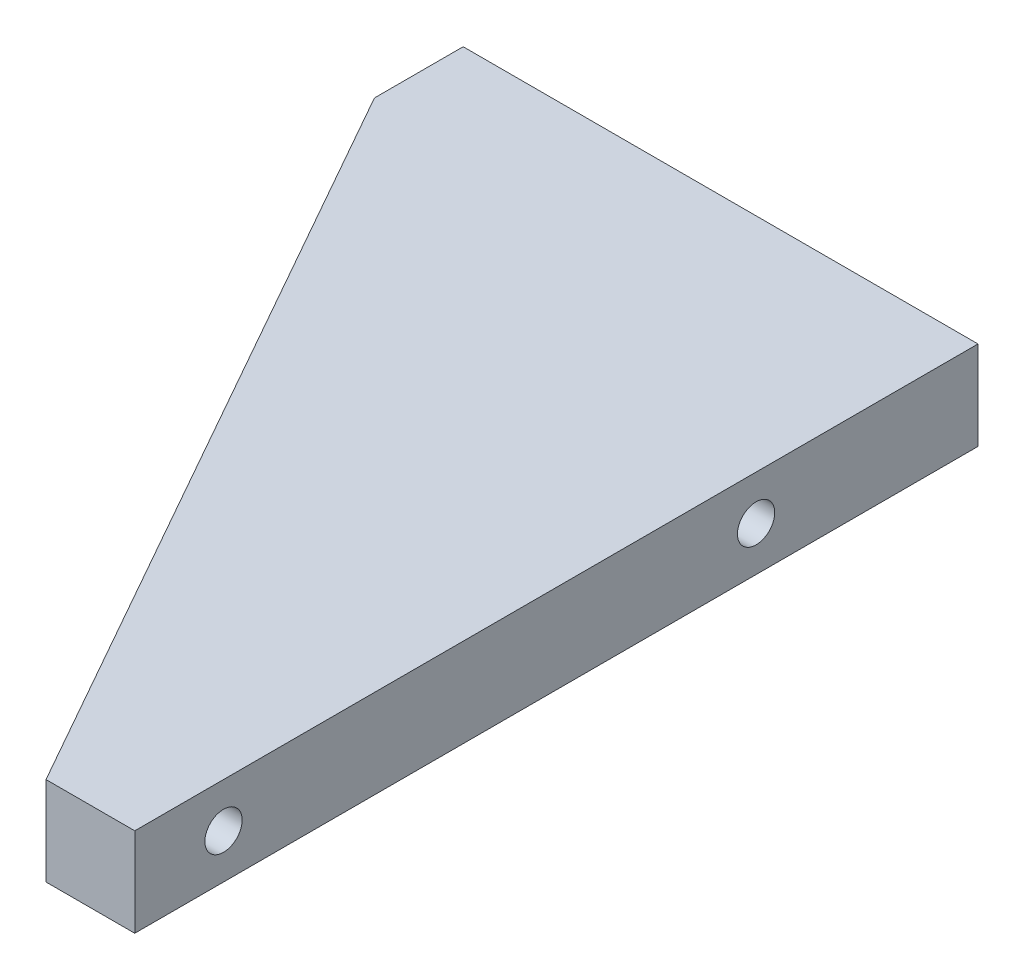
SolidWorks part; units mm, degrees
material "A6061"
ref_plane "前基準面" through (0, 0, 0) normal (0, 0, 1) x (1, 0, 0)
ref_plane "上基準面" through (0, 0, 0) normal (0, 1, 0) x (1, 0, 0)
ref_plane "右基準面" through (0, 0, 0) normal (1, 0, 0) x (0, 0, -1)
sketch "草图1" plane through (0, 0, 0) normal (0, 1, 0) x (1, 0, 0)
  line L1 (-29, -47.5) -> (29, -47.5)
  line L2 (-29, -47.5) -> (-29, 47.5)
  line L3 (-29, 47.5) -> (29, 47.5)
  line L4 (29, -47.5) -> (29, 47.5)
  line L5 (-29, -47.5) -> (29, 47.5) construction
  line L6 (-29, 47.5) -> (29, -47.5) construction
  point P0 (0, 0)
  dimension "D1" = 58
  dimension "D2" = 95
extrude "凸台-拉伸1" add sketch "草图1" along normal mid plane 10
sketch "草图2" plane through (0, 5, 0) normal (0, 1, 0) x (1, 0, 0)
  line L0 (19, -47.5) -> (-29, 37.5)
  line L1 (-29, -47.5) -> (29, -47.5) construction
  line L2 (-29, 47.5) -> (-29, -47.5) construction
  line L3 (-29, 37.5) -> (-29, -47.5)
  line L4 (-29, -47.5) -> (19, -47.5)
  line L5 (29, -47.5) -> (29, 47.5) construction
  line L6 (29, 47.5) -> (-29, 47.5) construction
  dimension "D1" = 10
  dimension "D2" = 10
extrude "切除-拉伸1" cut sketch "草图2" against normal up to surface (10 mm away) up to face at (0, -5, 0)
hole_wizard "M5 螺纹孔1" positions "草图3" profile "草图4" tap size "M5" standard "GB"
sketch "草图3" plane through (29, 0, 0) normal (1, 0, 0) x (0, 0, -1)
  line L0 (-47.5, 5) -> (-47.5, -5) construction
  point P0 (-37.5, 0)
  point P5 (22.5, 0)
  dimension "D2" = 10
  dimension "D3" = 60
  dimension "D1" = 2
sketch "草图4" plane through (29, 0, 37.5) normal (0, 1, 0) x (0, 0, -1)
  line L0 (0, 0) -> (0, 13.6618)
  line L1 (0, 13.6618) -> (2.1, 12.4)
  line L2 (2.1, 12.4) -> (2.1, 0)
  line L5 (2.1, 0) -> (0, 0)
  line L10 (0, 13.6618) -> (-2.1, 12.4) construction
  line L11 (0, -6.35) -> (0, 107.95) construction
  dimension "螺纹孔钻头直径" = 4.2
  dimension "螺纹孔钻头深度" = 12.4
  dimension "导头角度" = 118
cosmetic thread "孔螺蚊线1" parameters "D1"=10, "D2"=5
cosmetic thread "孔螺蚊线2" parameters "D1"=10, "D2"=5
hole_wizard "M5 螺纹孔2" positions "草图5" profile "草图6" tap size "M5" standard "GB"
sketch "草图5" plane through (0, 0, -47.5) normal (0, 0, -1) x (-1, 0, 0)
  line L0 (29, 5) -> (29, -5) construction
  point P0 (19, 0)
  point P2 (-21, 0)
  dimension "D1" = 40
  dimension "D2" = 10
sketch "草图6" plane through (-19, 0, -47.5) normal (1, 0, 0) x (0, 1, 0)
  line L0 (0, 0) -> (0, 13.6618)
  line L1 (0, 13.6618) -> (2.1, 12.4)
  line L2 (2.1, 12.4) -> (2.1, 0)
  line L5 (2.1, 0) -> (0, 0)
  line L10 (0, 13.6618) -> (-2.1, 12.4) construction
  line L11 (0, -6.35) -> (0, 107.95) construction
  dimension "螺纹孔钻头直径" = 4.2
  dimension "螺纹孔钻头深度" = 12.4
  dimension "导头角度" = 118
cosmetic thread "孔螺蚊线3" parameters "D1"=10, "D2"=5
cosmetic thread "孔螺蚊线4" parameters "D1"=10, "D2"=5
